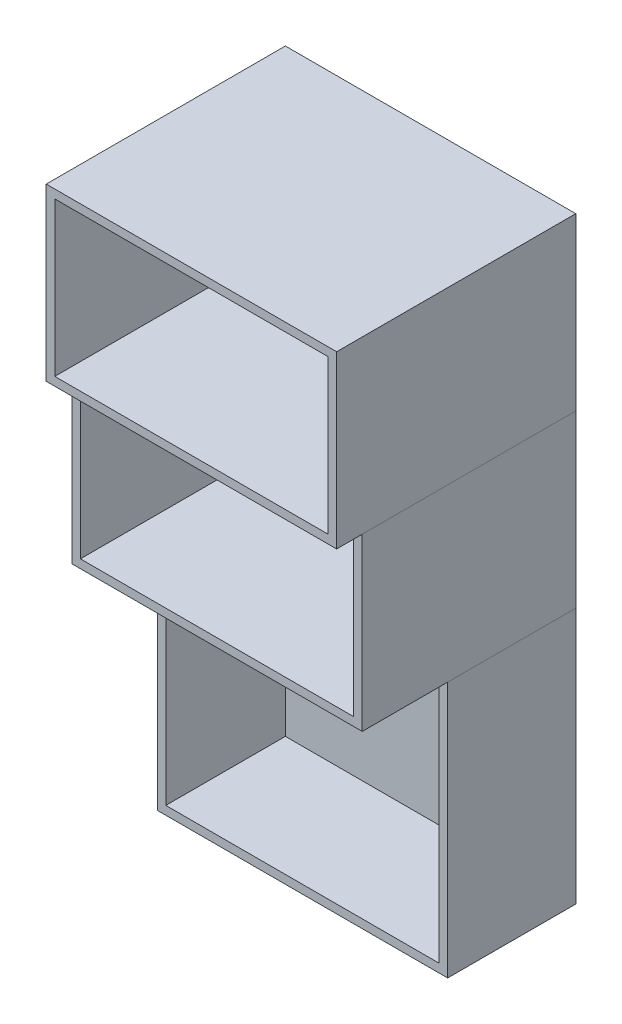
from build123d import *

# Parameters (mm, degrees)
SKETCH_1_W      = 340
SKETCH_1_H      = 200
EXTRUDE_1_DEPTH = 280
SHELL_1_T       = -10
SKETCH_2_W      = 340
SKETCH_2_H      = 200
EXTRUDE_2_DEPTH = 250
SHELL_2_T       = -10
SKETCH_3_W      = 340
SKETCH_3_H      = 300
EXTRUDE_3_DEPTH = 150
SHELL_3_T       = -10


with BuildPart() as part:
    # 草图1 → 凸台-拉伸1 (new body)
    with BuildSketch(Plane.XY):
        Rectangle(SKETCH_1_W, SKETCH_1_H)
    extrude(amount=EXTRUDE_1_DEPTH)

    # 抽壳1
    shell_1_openings = [part.faces().sort_by_distance(p)[0] for p in [
        (0, 0, 280),
    ]]
    offset(amount=SHELL_1_T, openings=shell_1_openings, kind=Kind.INTERSECTION)


with BuildPart() as body_2:
    # 草图2 → 凸台-拉伸2 (new body)
    with BuildSketch(Plane(origin=(0, 0, 0), x_dir=(-1, 0, 0), z_dir=(0, 0, -1))):
        with Locations((0, -200)):
            Rectangle(SKETCH_2_W, SKETCH_2_H)
    extrude(amount=-EXTRUDE_2_DEPTH)

    # 抽壳2
    shell_2_openings = [body_2.faces().sort_by_distance(p)[0] for p in [
        (0, -200, 250),
    ]]
    offset(amount=SHELL_2_T, openings=shell_2_openings, kind=Kind.INTERSECTION)


with BuildPart() as body_3:
    # 草图3 → 凸台-拉伸3 (new body)
    with BuildSketch(Plane(origin=(0, 0, 0), x_dir=(-1, 0, 0), z_dir=(0, 0, -1))):
        with Locations((0, -450)):
            Rectangle(SKETCH_3_W, SKETCH_3_H)
    extrude(amount=-EXTRUDE_3_DEPTH)

    # 抽壳3
    shell_3_openings = [body_3.faces().sort_by_distance(p)[0] for p in [
        (0, -450, 150),
    ]]
    offset(amount=SHELL_3_T, openings=shell_3_openings, kind=Kind.INTERSECTION)


solid = Compound([part.part, body_2.part, body_3.part])
